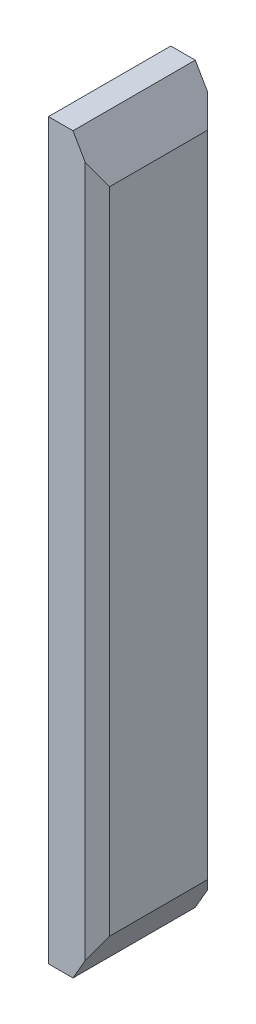
from build123d import *
from OCP.BRepFilletAPI import BRepFilletAPI_MakeChamfer

# Parameters (mm, degrees)
SKETCH_1_W      = 10
SKETCH_1_H      = 60
EXTRUDE_1_DEPTH = 4
CHAMFER_1_SIZE  = 2
CHAMFER_1_SIZE2 = 3.464101615
CHAMFER_2_SIZE  = 1


with BuildPart() as part:
    # 草图1 → 凸台-拉伸1 (new body)
    with BuildSketch(Plane(origin=(0, 0, 0), x_dir=(0, 0, -1), z_dir=(1, 0, 0))):
        Rectangle(SKETCH_1_W, SKETCH_1_H)
    extrude(amount=EXTRUDE_1_DEPTH)

    # 倒角1: one chamfer whose edges measure the first distance from different faces: ONE call of the kernel's chamfer builder (chamfer() names one face for all edges)
    chamfer_1_edges_1 = [part.edges().sort_by_distance(p)[0] for p in [
        (4, 30, 0),
    ]]
    chamfer_1_side_1 = [part.faces().sort_by_distance(p)[0] for p in [
        (2, 30, 0),
    ]]
    chamfer_1_edges_2 = [part.edges().sort_by_distance(p)[0] for p in [
        (4, -30, 0),
    ]]
    chamfer_1_side_2 = [part.faces().sort_by_distance(p)[0] for p in [
        (2, -30, 0),
    ]]
    chamfer_1 = BRepFilletAPI_MakeChamfer(part.part.solid().wrapped)
    for e in chamfer_1_edges_1:
        chamfer_1.Add(CHAMFER_1_SIZE, CHAMFER_1_SIZE2, e.wrapped, chamfer_1_side_1[0].wrapped)  # the first distance lies on this face
    for e in chamfer_1_edges_2:
        chamfer_1.Add(CHAMFER_1_SIZE, CHAMFER_1_SIZE2, e.wrapped, chamfer_1_side_2[0].wrapped)  # the first distance lies on this face
    add(Compound.cast(chamfer_1.Shape()), mode=Mode.REPLACE)

    # 倒角2
    chamfer_2_edges = [part.edges().sort_by_distance(p)[0] for p in [
        (4, 0, 5),
        (4, 0, -5),
    ]]
    chamfer(chamfer_2_edges, length=CHAMFER_2_SIZE)


solid = part.part
